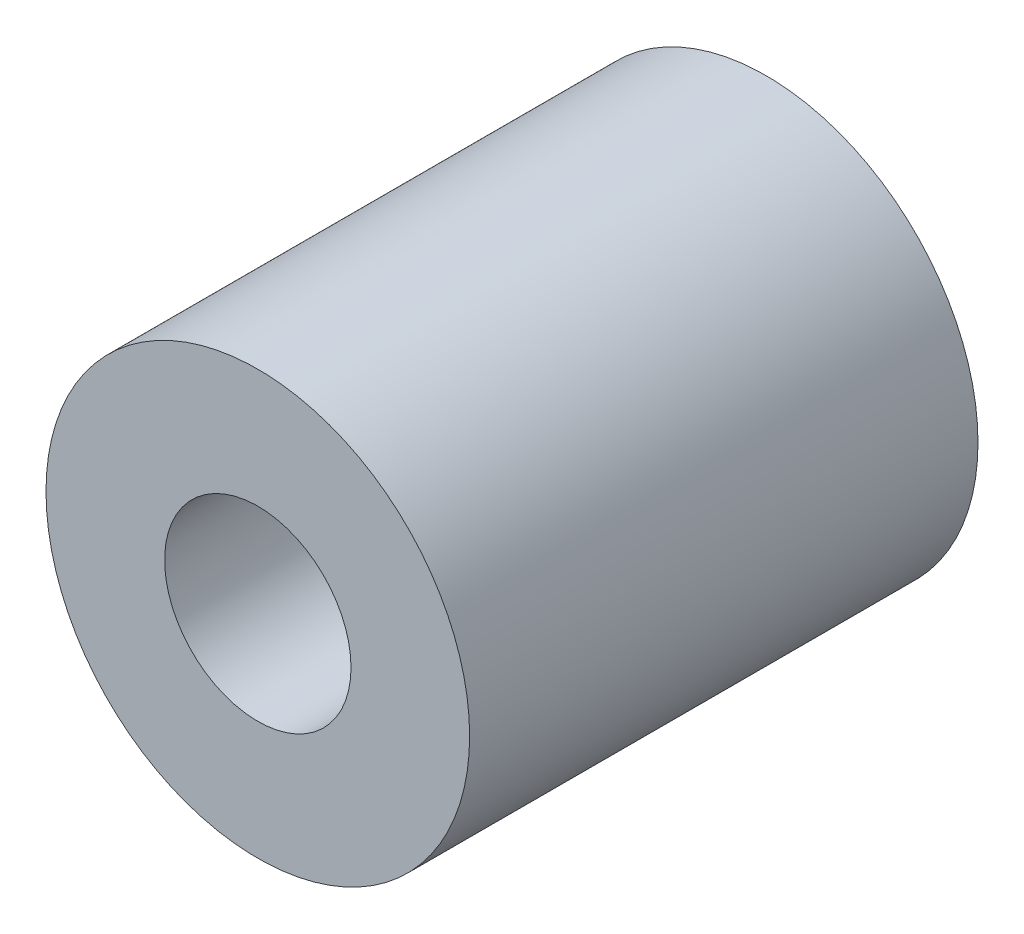
from build123d import *

# Parameters (mm, degrees)
SKETCH_1_R      = 5
SKETCH_1_R_2    = 2.2
EXTRUDE_1_DEPTH = 6


with BuildPart() as part:
    # 草图1 → 凸台-拉伸1 (new, symmetric)
    with BuildSketch(Plane.XY):
        Circle(SKETCH_1_R)
        Circle(SKETCH_1_R_2, mode=Mode.SUBTRACT)
    extrude(amount=EXTRUDE_1_DEPTH, both=True)


solid = part.part
